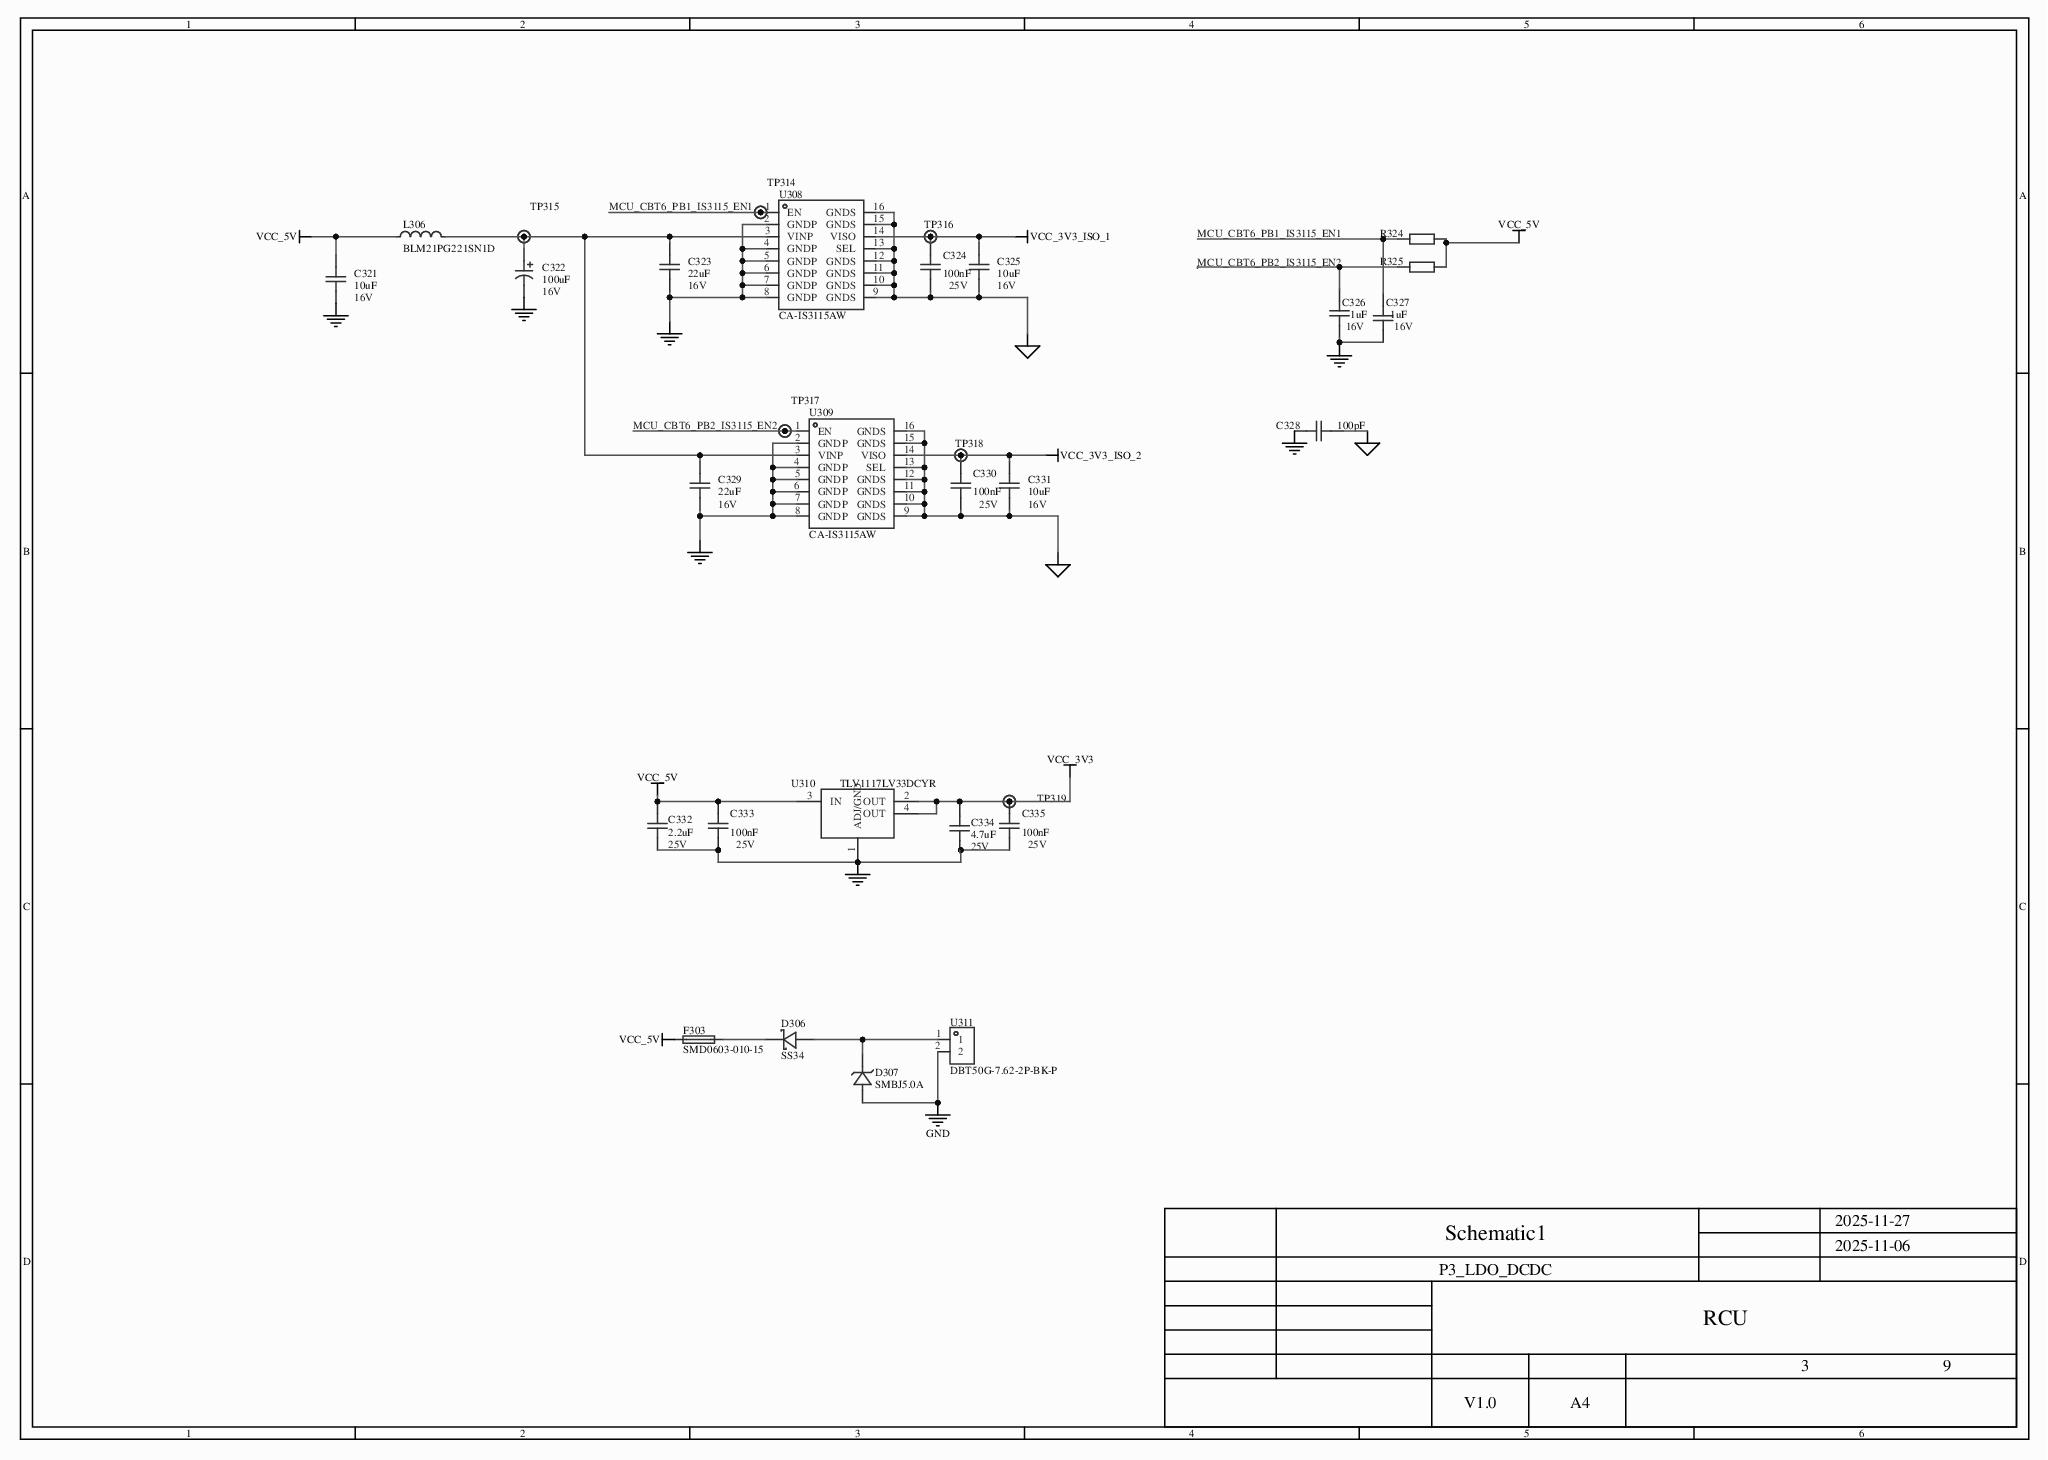
[diagram p0: MISC84429-4.SchDoc]
# Altium project MISC84429-12.PrjPcb (part 2 of 5)
## Sheet MISC84429-4.SchDoc (continued)
### Library data of the parts (continued)
TP314-TP319 = Test-Point: Add into BOM: yes; Symbol: Test-Point; Device: Test-Point; Convert to PCB: yes; Origin Footprint: Test-Point-0.5mm
U308 U309 = CA-IS3115AW: Add into BOM: yes; Output Power: 1.5W; Vin: 5V; Isolation voltage: 5kV; Symbol: CA-IS3115AW; Device: CA-IS3115AW; Supplier Part: C20598894; Manufacturer Part: CA-IS3115AW; Supplier Footprint: SOIC-16-WB; Datasheet: https://item.szlcsc.com/datasheet/CA-IS3115AW/21939206.html; Supplier: LCSC; Convert to PCB: yes; Origin Footprint: SOIC-16_L10.3-W7.5-P1.27-LS10.3-BL
U310 = TLV1117LV33DCYR: Add into BOM: yes; Maximum Input Voltage: 5.5V; Output Voltage: 3.3V; Output Current: 1A; Power Supply Rejection Ratio (PSRR): 75dB@(120Hz); Dropout Voltage: 1.3V@(800mA); standby current: 100uA; Number of Outputs: 1; Symbol: TLV1117LV33DCYR; Device: TLV1117LV33DCYR; Supplier Part: C15578; Manufacturer Part: TLV1117LV33DCYR; Supplier Footprint: SOT-223; Datasheet: https://www.ti.com/cn/lit/gpn/tlv1117lv; Supplier: LCSC; Convert to PCB: yes; Origin Footprint: SOT-223_L6.7-W3.5-P2.30-BR
U311 = DBT50G-7.62-2P-BK-P: Add into BOM: yes; Pitch: 7.62mm; Number of Positions or Pins: 1x2P; Number of PINs Per Row: 2; Current Rating: 20A; Voltage Rating (Max): 300V; Wire Gauge - AWG: 12~22; Symbol: DBT50G-7.62-2P-BK-P; Device: DBT50G-7.62-2P-BK-P; Supplier Part: C496127; Manufacturer Part: DBT50G-7.62-2P-BK-P; Datasheet: https://item.szlcsc.com/datasheet/DBT50G-7.62-2P-BK-P/507694.html; Supplier: LCSC; Convert to PCB: yes; Number of Pins: 2P; Number of Rows: 1; Wire Gauge - mm2: -; Origin Footprint: CONN-TH_2P-P7.62_L15.2-W16.7-EX4.2

## Sheet MISC84429-3.SchDoc
size 431 x 309 mm; Name: Sheet-Symbol; Symbol: Sheet-Symbol; Device: Sheet-Symbol; @Page No: 2; @Page Count: 9; @Schematic Name: 1_P1; @Project Name: Altium_Altium_RCU_2025-11-28_2026-01-14; @Board Name: 1_P1; @Update Date: 2026-01-15; @Create Time: 06:40:55; @Update Time: 14:40:57; @Page Name: 2_P2_POWER; @Create Date: 2026-01-15
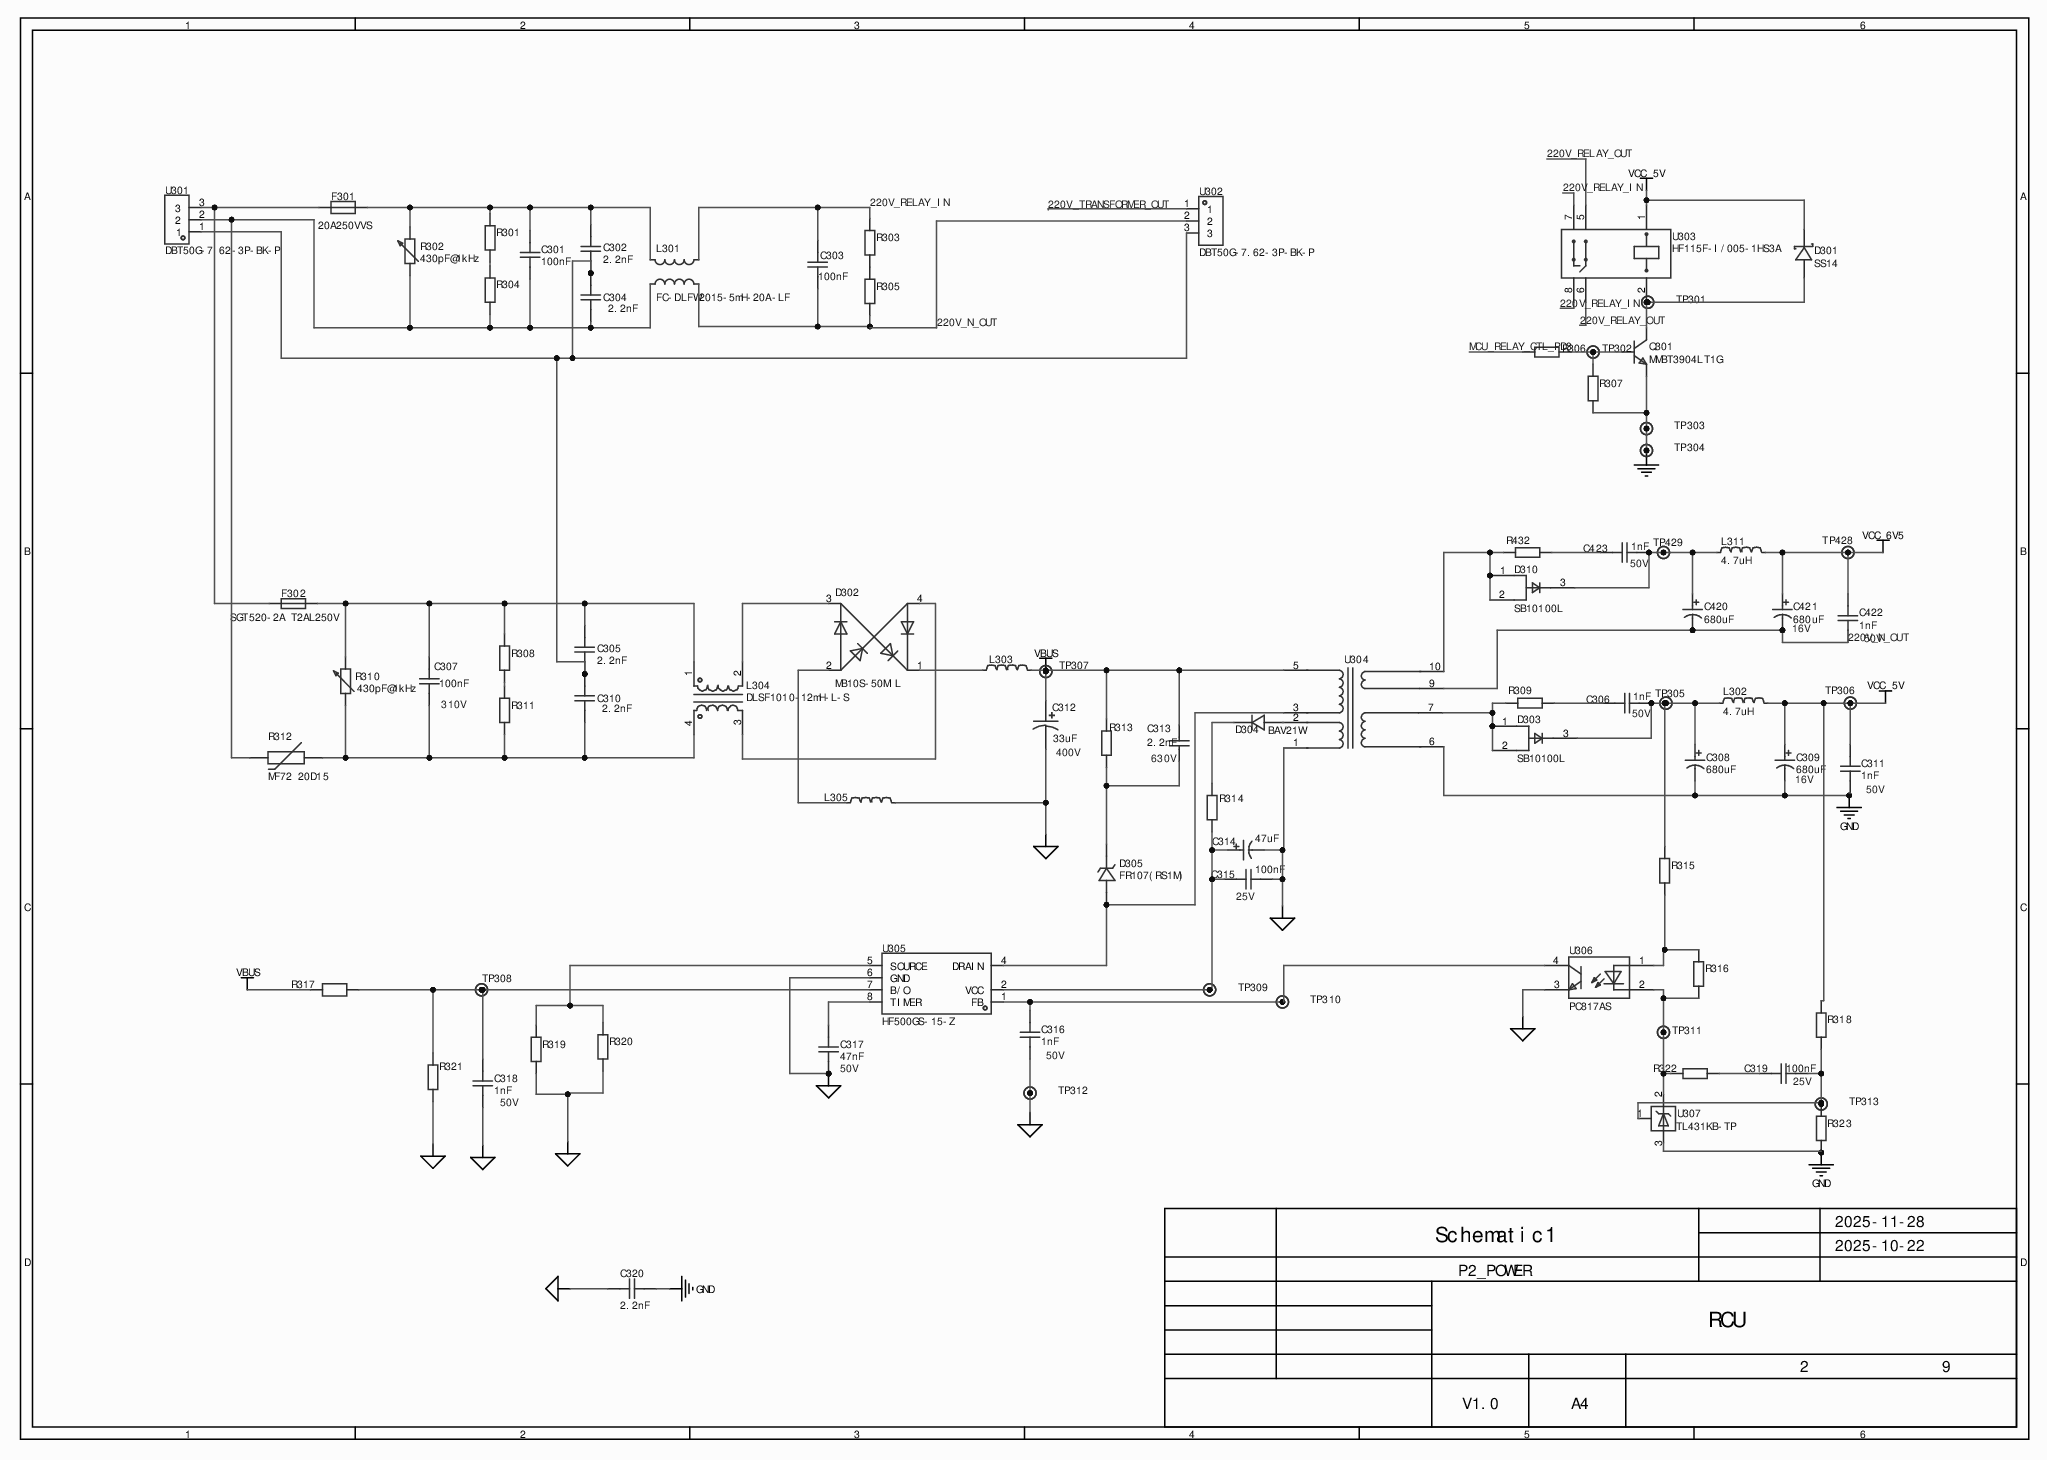
[diagram p1: MISC84429-3.SchDoc]

### Parts
C301  100nF  [CAP-TH_L13.0-W6.0-P10.00-D0.6]
C302  2.2nF  [CAP-TH_L8.0-W4.0-P7.50-D1.2]
C303  100nF  [CAP-TH_L13.0-W6.0-P10.00-D0.6]
C304  2.2nF  [CAP-TH_L8.0-W4.0-P7.50-D1.2]
C305  2.2nF  [CAP-TH_L8.0-W4.0-P7.50-D1.2]
C306  1nF  Voltage Rated: 50V  [C0603]
C307  100nF  Voltage(AC): 310V  [CAP-TH_L13.0-W6.0-P10.00-D0.6]
C308  680uF  [CAP-TH_BD8.0-P3.50-D0.6-FD]
C309  680uF  Voltage Rating: 16V  [CAP-TH_BD8.0-P3.50-D0.6-FD]
C310  2.2nF  [CAP-TH_L8.0-W4.0-P7.50-D1.2]
C311  1nF  Voltage Rated: 50V  [C0603]
C312  33uF  Voltage Rating: 400V  [CAP-TH_BD10.0-P5.00-D1.0-FD]
C313  2.2nF  Voltage Rating: 630V  [C1206]
C314  47uF  [CAP-TH_BD5.0-P2.00-D0.8-FD]
C315  100nF  Voltage Rated: 25V  [C0603]
C316  1nF  Voltage Rated: 50V  [C0603]
C317  47nF  Voltage Rated: 50V  [C0603]
C318  1nF  Voltage Rated: 50V  [C0603]
C319  100nF  Voltage Rated: 25V  [C0603]
C320  2.2nF  [CAP-TH_L10.0-W4.5-P10.00-D0.6-S4.0]
C420  680uF  [CAP-TH_BD8.0-P3.50-D0.6-FD]
C421  680uF  Voltage Rating: 16V  [CAP-TH_BD8.0-P3.50-D0.6-FD]
C422  1nF  Voltage Rated: 50V  [C0603]
C423  1nF  Voltage Rated: 50V  [C0603]
D301  SS14  [SMA_L4.3-W2.6-LS5.2-RD]
D302  MB10S-50MIL  [MBS_L4.7-W3.8-P2.40-LS7.0-TL]
D303  SB10100L  [TO-277A_L4.7-W6.1-LS6.6-TR]
D304  BAV21W  [SOD-123_L2.8-W1.8-LS3.7-RD]
D305  FR107(RS1M)  [SMA_L4.3-W2.6-LS5.2-RD]
D310  SB10100L  [TO-277A_L4.7-W6.1-LS6.6-TR]
F301  20A250VVS  [FUSE-TH_L8.4-W4.0-P5.08-D0.6]
F302  SGT520-2A T2AL250V  [FUSE-SMD_L20.0-W5.0]
L301  FC-DLFW2015-5mH-20A-LF  [FILTER-TH_FC-DLFW2015-5MH-20A-LF]
L302  4.7uH  [IND-SMD_L5.4-W5.2_FXL0530]
L303  (no value)  [L1206]
L304  DLSF1010-12mH-L-S  [IND-TH_4P-L14.0-W12.0_DLSF1010-12MH-L-S]
L305  (no value)  [L1206]
L311  4.7uH  [IND-SMD_L5.4-W5.2_FXL0530]
Q301  MMBT3904LT1G  [SOT-23-3_L2.9-W1.6-P1.90-LS2.8-BR]
R301  (no value)  [R1206]
R302  430pF@1kHz  [RES-TH_L16.5-W5.6-P7.50-D1.2-S3.00]
R303  (no value)  [R1206]
R304  (no value)  [R1206]
R305  (no value)  [R1206]
R306  (no value)  [R0603]
R307  (no value)  [R0603]
R308  (no value)  [R1206]
R309  (no value)  [R1206]
R310  430pF@1kHz  [RES-TH_L16.5-W5.6-P7.50-D1.2-S3.00]
R311  (no value)  [R1206]
R312  MF72 20D15  [RES-TH_L17.5-W6.0-P7.50-D0.8-S7.50]
R313  (no value)  [R1206]
R314  (no value)  [R1206]
R315  (no value)  [R0603]
R316  (no value)  [R0603]
R317  (no value)  [R1206]
R318  (no value)  [R0603]
R319  (no value)  [R1206]
R320  (no value)  [R1206]
R321  (no value)  [R0603]
R322  (no value)  [R0603]
R323  (no value)  [R0603]
R432  (no value)  [R1206]
TP301  (no value)  [Test-Point-0.5mm]
TP302  (no value)  [Test-Point-0.5mm]
TP303  (no value)  [Test-Point-0.5mm]
TP304  (no value)  [Test-Point-0.5mm]
TP305  (no value)  [Test-Point-0.5mm]
TP306  (no value)  [Test-Point-0.5mm]
TP307  (no value)  [Test-Point-0.5mm]
TP308  (no value)  [Test-Point-0.5mm]
TP309  (no value)  [Test-Point-0.5mm]
TP310  (no value)  [Test-Point-0.5mm]
TP311  (no value)  [Test-Point-0.5mm]
TP312  (no value)  [Test-Point-0.5mm]
TP313  (no value)  [Test-Point-0.5mm]
TP428  (no value)  [Test-Point-0.5mm]
TP429  (no value)  [Test-Point-0.5mm]
U301  DBT50G-7.62-3P-BK-P  [CONN-TH_3P-P7.62_L15.2-W24.4-EX4.2]
U302  DBT50G-7.62-3P-BK-P  [CONN-TH_3P-P7.62_L15.2-W24.4-EX4.2]
U303  HF115F-I/005-1HS3A  [RELAY-TH_HF115F-XXX-1HS3]
U304  (no value)  [111]
U305  HF500GS-15-Z  [SOIC-8_7P-L4.9-W3.9-P1.27-LS6.0-BL-PE3]
U306  PC817AS  [SOP-4_L6.5-W4.6-P2.54-LS10.2-TL]
U307  TL431KB-TP  [SOT-23-3_L2.9-W1.4-P1.91-LS2.6-BR]

### Nets
AGND: C312.2 C314.2 C315.2 C316.1 C317.1 C318.1 C320.1 L305.2 R319.1 R320.1 R321.1 TP312.1 U304.1 U305.6(GND) U306.3(CAT)
GND: C308.2 C309.2 C311.1 C320.2 Q301.2 R307.2 R323.1 TP303.1 TP304.1 U304.6 U307.3(-)
VBUS: C312.1 C313.2 L303.2 R313.2 R317.1 TP307.1 U304.5
VCC_5V: C309.1 C311.2 D301.1(K) L302.2 R318.2 TP306.1 U303.1
VCC_6V5: C421.1 C422.2 L311.2 TP428.1
220V_N_OUT: C303.1 C420.2 C421.2 C422.1 L301.4 R305.1 U302.2 U304.9
220V_RELAY_IN: C303.2 L301.3 R303.2 U303.7 U303.8
220V_RELAY_OUT: U303.5 U303.6
220V_TRANSFORMER_OUT: U302.1
MCU_RELAY_CTL_PD3: R306.1
NetC301_1: C301.1 C304.1 L301.1 R302.1 R304.1 R312.1 U301.2
NetC301_2: C301.2 C302.2 F301.2 L301.2 R301.2 R302.2
NetC302_1: C302.1 C304.2 C305.1 C310.2 U301.1 U302.3
NetC305_2: C305.2 C307.2 F302.2 L304.1 R308.2 R310.2
NetC306_1: C306.1 C308.1 D303.3 L302.1 R315.2 TP305.1
NetC306_2: C306.2 R309.2
NetC307_1: C307.1 C310.1 L304.4 R310.1 R311.1 R312.2
NetC313_1: C313.1 D305.1(C) R313.1
NetC314_1: C314.1 C315.1 R314.1 TP309.1 U305.2(VCC)
NetC316_2: C316.2 TP310.1 U305.1(FB) U306.4(AN)
NetC317_2: C317.2 U305.8(TIMER)
NetC318_2: C318.2 R317.2 R321.2 TP308.1 U305.7(B/O)
NetC319_1: C319.1 R322.2
NetC319_2: C319.2 R318.1 R323.2 TP313.1 U307.1(REF)
NetC420_1: C420.1 C423.1 D310.3 L311.1 TP429.1
NetC423_2: C423.2 R432.2
NetD301_2: D301.2(A) Q301.3 TP301.1 U303.2
NetD302_1: D302.1(+) L303.1
NetD302_2: D302.2(-) L305.1
NetD302_3: D302.3(C2) L304.2
NetD302_4: D302.4(C1) L304.3
NetD303_1: D303.1 D303.2 R309.1 U304.7
NetD304_1: D304.1(K) R314.2
NetD304_2: D304.2(A) U304.2
NetD305_2: D305.2(A) U304.3 U305.4(DRAIN)
NetD310_1: D310.1 D310.2 R432.1 U304.10
NetF301_1: F301.1 F302.1 U301.3
NetQ301_1: Q301.1 R306.2 R307.1 TP302.1
NetR301_1: R301.1 R304.2
NetR303_1: R303.1 R305.2
NetR308_1: R308.1 R311.2
NetR315_1: R315.1 R316.2 U306.1(COL)
NetR316_1: R316.1 R322.1 TP311.1 U306.2(EM) U307.2(+)
NetR319_2: R319.2 R320.2 U305.5(SOURCE)

### Notes on the sheet
- 1
- 2
- 3
- 4
- 5
- 6
- A
- B
- C
- D
- Schematic1
- 2025-11-28
- 2025-10-22
- P2_POWER
- RCU
- 9
- V1.0
- A4

### Library data of the parts
C301 C303 C307 = 100nF: Symbol: MPX104K31C3KN15600; Add into BOM: yes; Ratings: X2; Device: 100nF; Supplier Part: C489079; Manufacturer Part: MPX104K31C3KN15600; Datasheet: https://atta.szlcsc.com/upload/public/pdf/source/20200225/C489079_75CB6A5338414DC85C4C6073302579B5.pdf; Supplier: LCSC; Convert to PCB: yes; Value: 100nF; Origin Footprint: CAP-TH_L13.0-W6.0-P10.00-D0.6; Design Item ID: MPX104K31C3KN15600
C302 C304 C305 C310 = 2.2nF: Symbol: G08F1E222MN0B0S0N0; Add into BOM: yes; Voltage(AC): 250V; Ratings: Y2; Device: 2.2nF; Supplier Part: C240878; Manufacturer Part: G08F1E222MN0B0S0N0; Datasheet: https://item.szlcsc.com/datasheet/G08F1E222MN0B0S0N0/239854.html; Supplier: LCSC; Convert to PCB: yes; Value: 2.2nF; Origin Footprint: CAP-TH_L8.0-W4.0-P7.50-D1.2; Design Item ID: G08F1E222MN0B0S0N0
C306 C311 C316 C318 C422 C423 = 1nF: Symbol: GRM188R71H102KA01D; Add into BOM: yes; Temperature Coefficient: X7R; Device: 1nF; Supplier Part: C71653; Manufacturer Part: GRM188R71H102KA01D; Supplier Footprint: 0603; Datasheet: https://atta.szlcsc.com/upload/public/pdf/source/20161108/1478586450384.pdf; Supplier: LCSC; Convert to PCB: yes; Value: 1nF; Origin Footprint: C0603; Design Item ID: GRM188R71H102KA01D
C308 C420 = 680uF: Symbol: ULR687M1CF1ARR; Add into BOM: yes; Voltage Rating: 16V; Ripple Current: 5.1A@100kHz; Pin Spacing: 3.5mm; Device: 680uF; Supplier Part: C248458; Manufacturer Part: ULR687M1CF1ARR; Datasheet: https://atta.szlcsc.com/upload/public/pdf/source/20181106/C248463_8FFE85A6B0231DD342132C712786FADC.pdf; Supplier: LCSC; Convert to PCB: yes; Value: 680uF; Type: -; Diameter: 8mm; Height - Seated (Max): 11.5mm; Origin Footprint: CAP-TH_BD8.0-P3.50-D0.6-FD; Design Item ID: ULR687M1CF1ARR
C309 C421 = 680uF: Symbol: ULR687M1CF1ARR; Add into BOM: yes; Ripple Current: 5.1A@100kHz; Pin Spacing: 3.5mm; Device: 680uF; Supplier Part: C248458; Manufacturer Part: ULR687M1CF1ARR; Datasheet: https://atta.szlcsc.com/upload/public/pdf/source/20181106/C248463_8FFE85A6B0231DD342132C712786FADC.pdf; Supplier: LCSC; Convert to PCB: yes; Value: 680uF; Type: -; Diameter: 8mm; Height - Seated (Max): 11.5mm; Origin Footprint: CAP-TH_BD8.0-P3.50-D0.6-FD; Design Item ID: ULR687M1CF1ARR
C312 = 33uF: Symbol: 87EC0179; Add into BOM: yes; Ripple Current: 440mA@120Hz; Pin Spacing: 5mm; Device: 33uF; Supplier Part: C516822; Manufacturer Part: 87EC0179; Datasheet: https://item.szlcsc.com/datasheet/87EC0179/533670.html; Supplier: LCSC; Convert to PCB: yes; Value: 33uF; Equivalent Series Resistance(ESR): -; Diameter: 10mm; Height - Seated (Max): 18mm; Origin Footprint: CAP-TH_BD10.0-P5.00-D1.0-FD; Design Item ID: 87EC0179
C313 = 2.2nF: Symbol: GRM31BR72J222KW01L; Add into BOM: yes; Temperature Coefficient: X7R; Device: 2.2nF; Supplier Part: C97938; Manufacturer Part: GRM31BR72J222KW01L; Supplier Footprint: 1206; Datasheet: https://item.szlcsc.com/datasheet/GRM31BR72J222KW01L/99147.html; Supplier: LCSC; Convert to PCB: yes; Value: 2.2nF; Origin Footprint: C1206; Design Item ID: GRM31BR72J222KW01L
C314 = 47uF: Symbol: KS476M025D07RR0VH2FP0; Add into BOM: yes; Voltage Rating: 25V; Pin Spacing: 2mm; Device: 47uF; Supplier Part: C44586; Manufacturer Part: KS476M025D07RR0VH2FP0; Datasheet: https://item.szlcsc.com/datasheet/KS476M025D07RR0VH2FP0/45588.html; Supplier: LCSC; Convert to PCB: yes; Value: 47uF; Diameter: 5mm; Height - Seated (Max): 7mm; Origin Footprint: CAP-TH_BD5.0-P2.00-D0.8-FD; Design Item ID: KS476M025D07RR0VH2FP0
C315 C319 = 100nF: Symbol: GRM188R71E104KA01D; Add into BOM: yes; Temperature Coefficient: X7R; Device: 100nF; Supplier Part: C77050; Manufacturer Part: GRM188R71E104KA01D; Supplier Footprint: 0603; Datasheet: https://atta.szlcsc.com/upload/public/pdf/source/20170622/1498103881034.pdf; Supplier: LCSC; Convert to PCB: yes; Value: 100nF; Origin Footprint: C0603; Design Item ID: GRM188R71E104KA01D
C317 = 47nF: Symbol: GCJ188R71H473KA12D; Add into BOM: yes; Temperature Coefficient: X7R; Device: 47nF; Supplier Part: C354386; Manufacturer Part: GCJ188R71H473KA12D; Supplier Footprint: 0603; Datasheet: https://atta.szlcsc.com/upload/public/pdf/source/20190214/C354386_A23112F67A0EA363A33264332A959C51.pdf; Supplier: LCSC; Convert to PCB: yes; Value: 47nF; Origin Footprint: C0603; Design Item ID: GCJ188R71H473KA12D
C320 = 2.2nF: Symbol: AJTF222M2GF0200A082E; Add into BOM: yes; Voltage(AC): 400V; Ratings: Y1; Device: 2.2nF; Supplier Part: C2836435; Manufacturer Part: AJTF222M2GF0200A082E; Datasheet: https://item.szlcsc.com/datasheet/AJTF222M2GF0200A082E/3002607.html; Supplier: LCSC; Convert to PCB: yes; Value: 2.2nF; Origin Footprint: CAP-TH_L10.0-W4.5-P10.00-D0.6-S4.0; Design Item ID: AJTF222M2GF0200A082E
D301 = SS14: Symbol: SS14_C83852; Add into BOM: yes; Voltage - Forward(Vf@If): 500mV@1A; Voltage - DC Reverse(Vr): 40V; Current - Rectified: 1A; Reverse Leakage Current (Ir): 200uA@40V; Non-Repetitive Peak Forward Surge Current: 40A; Device: SS14; Supplier Part: C83852; Manufacturer Part: SS14; Supplier Footprint: SMA(DO-214AC); Datasheet: https://item.szlcsc.com/datasheet/SS14/85019.html; Supplier: LCSC; Convert to PCB: yes; Origin Footprint: SMA_L4.3-W2.6-LS5.2-RD; Design Item ID: SS14_C83852
D302 = MB10S-50MIL: Add into BOM: yes; Voltage - Forward(Vf@If): 1.1V@400mA; Voltage - DC Reverse(Vr): 1kV; Current - Rectified: 1A; Reverse Leakage Current (Ir): 5uA@1kV; Non-Repetitive Peak Forward Surge Current: 35A; Symbol: MB10S-50MIL; Device: MB10S-50MIL; Supplier Part: C2488; Manufacturer Part: MB10S-50MIL; Supplier Footprint: MBS; Datasheet: https://item.szlcsc.com/datasheet/MB10S-50MIL/2865.html; Supplier: LCSC; Convert to PCB: yes; Origin Footprint: MBS_L4.7-W3.8-P2.40-LS7.0-TL; Design Item ID: MB10S-50MIL
D303 D310 = SB10100L: Symbol: SB10100L_C113946; Add into BOM: yes; Voltage - Forward(Vf@If): 850mV@10A; Voltage - DC Reverse(Vr): 100V; Current - Rectified: 10A; Reverse Leakage Current (Ir): 300uA@100V; Non-Repetitive Peak Forward Surge Current: 150A; Device: SB10100L; Supplier Part: C113946; Manufacturer Part: SB10100L; Supplier Footprint: TO-277; Datasheet: https://item.szlcsc.com/datasheet/SB10100L/115185.html; Supplier: LCSC; Convert to PCB: yes; Origin Footprint: TO-277A_L4.7-W6.1-LS6.6-TR; Design Item ID: SB10100L_C113946
D304 = BAV21W: Symbol: BAV21W_C113947; Add into BOM: yes; Voltage - Forward(Vf@If): 1.25V@200mA; Voltage - DC Reverse(Vr): 250V; Current - Rectified: 200mA; Pd - Power Dissipation: 500mW; Reverse Leakage Current (Ir): 100nA@250V; Reverse Recovery Time (trr): 50ns; Non-Repetitive Peak Forward Surge Current: 3A; Device: BAV21W; LCSC Part Name: BAV21W; Supplier Part: C113947; Manufacturer Part: BAV21W; Supplier Footprint: SOD-123; Datasheet: https://item.szlcsc.com/datasheet/BAV21W/115186.html; Supplier: LCSC; Convert to PCB: yes; Origin Footprint: SOD-123_L2.8-W1.8-LS3.7-RD; Design Item ID: BAV21W_C113947
D305 = FR107(RS1M): Add into BOM: yes; Voltage - Forward(Vf@If): 1.3V@1A; Voltage - DC Reverse(Vr): 1kV; Current - Rectified: 1A; Reverse Leakage Current (Ir): 5uA; Reverse Recovery Time (trr): 500ns; Non-Repetitive Peak Forward Surge Current: 30A; Symbol: FR107(RS1M); Device: FR107(RS1M); Supplier Part: C489136; Manufacturer Part: FR107(RS1M); Supplier Footprint: DO-214AC(SMA); Datasheet: https://item.szlcsc.com/datasheet/FR107(RS1M)/499160.html; Supplier: LCSC; Convert to PCB: yes; Operating Junction Temperature Range: -; Origin Footprint: SMA_L4.3-W2.6-LS5.2-RD; Design Item ID: FR107(RS1M)
F301 = 20A250VVS: Symbol: MTS2200A; Add into BOM: yes; Current Rating: 20A; Voltage Rating (DC): 250V; Melting I2t: 960; Interrupt Rating: 35A@250VAC; Pitch: 5.08mm; Device: 20A250VVS; Supplier Part: C2762416; Manufacturer Part: 20A250VVS; Datasheet: https://item.szlcsc.com/datasheet/MTS2200A/2889372.html; Supplier: LCSC; Convert to PCB: yes; Origin Footprint: FUSE-TH_L8.4-W4.0-P5.08-D0.6; Design Item ID: MTS2200A
F302 = SGT520-2A T2AL250V: Add into BOM: yes; Current Rating: 2A; Voltage Rating (AC): 250V; Interrupt Rating: 35A@250VAC; Symbol: SGT520-2A T2AL250V; Device: SGT520-2A T2AL250V; Supplier Part: C2997153; Manufacturer Part: SGT520-2A T2AL250V; Supplier Footprint: D5xL20mm; Datasheet: https://atta.szlcsc.com/upload/public/pdf/source/20220512/3B2013244E644EF8C6E398858F77344C.pdf; Supplier: LCSC; Convert to PCB: yes; Origin Footprint: FUSE-SMD_L20.0-W5.0; Design Item ID: SGT520-2A T2AL250V
L301 = FC-DLFW2015-5mH-20A-LF: Add into BOM: yes; Number of Lines: 2; Withstanding Voltage: 1.5kV; Current Rating: 20A; Inductance @ Frequency: 5mH@1KHz; Symbol: FC-DLFW2015-5mH-20A-LF; Device: FC-DLFW2015-5mH-20A-LF; Supplier Part: C28314498; Manufacturer Part: FC-DLFW2015-5mH-20A-LF; Datasheet: https://atta.szlcsc.com/upload/public/pdf/source/20240808/62DBB3E748F582D3D16D94FF73003319.pdf; Supplier: LCSC; Convert to PCB: yes; Voltage Rating: -; Origin Footprint: FILTER-TH_FC-DLFW2015-5MH-20A-LF; Design Item ID: FC-DLFW2015-5mH-20A-LF
L302 L311 = 4.7uH: Symbol: FXL0530-4R7-M; Add into BOM: yes; Current Rating: 4.5A; Current - Saturation(Isat): 5A; Device: 4.7uH; Supplier Part: C177246; Manufacturer Part: FXL0530-4R7-M; Supplier Footprint: SMD,5.4x5.2mm; Datasheet: https://item.szlcsc.com/datasheet/FXL0530-4R7-M/188638.html; Supplier: LCSC; Convert to PCB: yes; Value: 4.7uH; Origin Footprint: IND-SMD_L5.4-W5.2_FXL0530; Design Item ID: FXL0530-4R7-M
L303 L305 = FCM3216KF-500T05: Add into BOM: yes; Current Rating: 500mA; Number of Circuits: 1; Symbol: FCM3216KF-500T05; Device: FCM3216KF-500T05; Supplier Part: C155098; Supplier Footprint: 1206; Datasheet: https://item.szlcsc.com/datasheet/FCM3216KF-500T05/166440.html; Supplier: LCSC; Convert to PCB: yes; Origin Footprint: L1206; Design Item ID: FCM3216KF-500T05
L304 = DLSF1010-12mH-L-S: Add into BOM: yes; Number of Lines: 2; Voltage Withstand: 1.5kV@AC,1mins; Inductance @ Frequency: 12mH@1kHz; Symbol: DLSF1010-12mH-L-S; Device: DLSF1010-12mH-L-S; Supplier Part: C2936077; Manufacturer Part: DLSF1010-12mH-L-S; Datasheet: https://item.szlcsc.com/datasheet/DLSF1010-12mH-L-S/3287820.html; Supplier: LCSC; Convert to PCB: yes; Origin Footprint: IND-TH_4P-L14.0-W12.0_DLSF1010-12MH-L-S; Design Item ID: DLSF1010-12mH-L-S
Q301 = MMBT3904LT1G: Add into BOM: yes; type: NPN; Current - Collector(Ic): 200mA; Collector - Emitter Voltage VCEO: 40V; Pd - Power Dissipation: 225mW; DC Current Gain: 40@0.1mA,1.0V; Transition frequency(fT): 300MHz; Current - Collector Cutoff: 50nA; Vce Saturation(VCE(sat)): 200mV; Symbol: MMBT3904LT1G; Device: MMBT3904LT1G; Supplier Part: C81464; Manufacturer Part: MMBT3904LT1G; Supplier Footprint: SOT-23; Datasheet: https://item.szlcsc.com/datasheet/MMBT3904LT1G/82615.html; Supplier: LCSC; Convert to PCB: yes; Origin Footprint: SOT-23-3_L2.9-W1.6-P1.90-LS2.8-BR; Design Item ID: MMBT3904LT1G
R301 R303-R305 R308 R311 = RC1206FR-07470KL: Add into BOM: yes; Power(Watts): 250mW; Voltage-Supply(Max): 200V; Symbol: RC1206FR-07470KL; Device: RC1206FR-07470KL; Supplier Part: C137273; Manufacturer Part: RC1206FR-07470KL; Supplier Footprint: 1206; Datasheet: https://item.szlcsc.com/datasheet/RC1206FR-07470KL/148589.html; Supplier: LCSC; Convert to PCB: yes; Origin Footprint: R1206; Design Item ID: RC1206FR-07470KL
R302 R310 = 430pF@1kHz: Symbol: 471KD14; Add into BOM: yes; Varistor Voltage: 470V; Clamping Voltage: 775V; Maximum DC Volts: 385V; Maximum AC Volts: 300V; Peak Current: 6kA; Energy: 175J; Rated Wattage: 600mW; Device: 430pF@1kHz; Supplier Part: C78353; Manufacturer Part: 471KD14; Datasheet: https://item.szlcsc.com/datasheet/471KD14/79488.html; Supplier: LCSC; Convert to PCB: yes; Value: 430pF@1kHz; Origin Footprint: RES-TH_L16.5-W5.6-P7.50-D1.2-S3.00; Design Item ID: 471KD14
R306 R315 = RC0603FR-071KL: Add into BOM: yes; Power(Watts): 100mW; Voltage-Supply(Max): 75V; Symbol: RC0603FR-071KL; Device: RC0603FR-071KL; Supplier Part: C22548; Manufacturer Part: RC0603FR-071KL; Supplier Footprint: 0603; Datasheet: https://atta.szlcsc.com/upload/public/pdf/source/20180316/70C0E2BDAE7FCC62C531A5A58D202EE1.pdf; Supplier: LCSC; Convert to PCB: yes; Origin Footprint: R0603; Design Item ID: RC0603FR-071KL
R307 = RC0603FR-07100KL: Add into BOM: yes; Power(Watts): 100mW; Overload Voltage (Max): 75V; Symbol: RC0603FR-07100KL; Device: RC0603FR-07100KL; Supplier Part: C14675; Manufacturer Part: RC0603FR-07100KL; Supplier Footprint: 0603; Datasheet: https://atta.szlcsc.com/upload/public/pdf/source/20140324/1457707028752.pdf; Supplier: LCSC; Convert to PCB: yes; Origin Footprint: R0603; Design Item ID: RC0603FR-07100KL
R309 R432 = RC1206FR-0722RL: Add into BOM: yes; Power(Watts): 250mW; Voltage-Supply(Max): 200V; Symbol: RC1206FR-0722RL; Device: RC1206FR-0722RL; Supplier Part: C114943; Manufacturer Part: RC1206FR-0722RL; Supplier Footprint: 1206; Datasheet: https://item.szlcsc.com/datasheet/RC1206FR-0722RL/116187.html; Supplier: LCSC; Convert to PCB: yes; Origin Footprint: R1206; Design Item ID: RC1206FR-0722RL
R312 = MF72 20D15: Add into BOM: yes; Steady State Current (Max): 4A; Thermal Time Constant: 43s; Pitch: 7.5mm; Symbol: MF72 20D15; Device: MF72 20D15; Supplier Part: C110642; Manufacturer Part: MF72 20D15; Datasheet: https://item.szlcsc.com/datasheet/MF72%252020D15/111867.html; Supplier: LCSC; Convert to PCB: yes; _1: -; _2: -; _3: -; _4: -; Power(Watts): -; B Constant Tolerance: -; Origin Footprint: RES-TH_L17.5-W6.0-P7.50-D0.8-S7.50; Design Item ID: MF72 20D15
R313 = RC1206FR-07150KL: Add into BOM: yes; Power(Watts): 250mW; Voltage-Supply(Max): 200V; Symbol: RC1206FR-07150KL; Device: RC1206FR-07150KL; Supplier Part: C114931; Manufacturer Part: RC1206FR-07150KL; Supplier Footprint: 1206; Datasheet: https://item.szlcsc.com/datasheet/RC1206FR-07150KL/116175.html; Supplier: LCSC; Convert to PCB: yes; Origin Footprint: R1206; Design Item ID: RC1206FR-07150KL
R314 = RC1206JR-0710RL: Add into BOM: yes; Power(Watts): 250mW; Voltage-Supply(Max): 200V; Symbol: RC1206JR-0710RL; Device: RC1206JR-0710RL; Supplier Part: C137208; Manufacturer Part: RC1206JR-0710RL; Supplier Footprint: 1206; Datasheet: https://item.szlcsc.com/datasheet/RC1206JR-0710RL/148524.html; Supplier: LCSC; Convert to PCB: yes; Origin Footprint: R1206; Design Item ID: RC1206JR-0710RL
R316 = RK73H1JTTD2001F: Manufacturer: KOA; Add into BOM: yes; Power(Watts): 100mW; Overload Voltage (Max): 75V; Symbol: RK73H1JTTD2001F; Device: RK73H1JTTD2001F; Supplier Part: C160026; Manufacturer Part: RK73H1JTTD2001F; Supplier Footprint: 0603; Datasheet: https://atta.szlcsc.com/upload/public/pdf/source/20190516/C346145_73DC9C40D36D5A63BE57BD2EFB7F1781.pdf; Supplier: LCSC; Convert to PCB: yes; Origin Footprint: R0603; Design Item ID: RK73H1JTTD2001F
R317 = 1206W4F1025T5E: Add into BOM: yes; Power(Watts): 250mW; Overload Voltage (Max): 200V; Symbol: 1206W4F1025T5E; Device: 1206W4F1025T5E; Supplier Part: C422611; Manufacturer Part: 1206W4F1025T5E; Supplier Footprint: 1206; Datasheet: https://atta.szlcsc.com/upload/public/pdf/source/20200306/C422600_1E6D84923E4A46A82E41ADD87F860B5C.pdf; Supplier: LCSC; Convert to PCB: yes; Origin Footprint: R1206; Design Item ID: 1206W4F1025T5E
R318 R322 R323 = RC0603FR-0710KL: as R324 on sheet MISC84429-4; Symbol: RC0603FR-0710KL; Device: RC0603FR-0710KL; Supplier Part: C98220; Manufacturer Part: RC0603FR-0710KL; Supplier Footprint: 0603; Datasheet: https://atta.szlcsc.com/upload/public/pdf/source/20180927/C295883_E8D83085EA81BD7DE0B2B681138C15EE.pdf; Supplier: LCSC; Convert to PCB: yes; Origin Footprint: R0603; Design Item ID: RC0603FR-0710KL
R319 R320 = RC1206FR-073R3L: Add into BOM: yes; Power(Watts): 250mW; Voltage-Supply(Max): 200V; Symbol: RC1206FR-073R3L; Device: RC1206FR-073R3L; Supplier Part: C137283; Manufacturer Part: RC1206FR-073R3L; Supplier Footprint: 1206; Datasheet: https://item.szlcsc.com/datasheet/RC1206FR-073R3L/148599.html; Supplier: LCSC; Convert to PCB: yes; Origin Footprint: R1206; Design Item ID: RC1206FR-073R3L
R321 = RC0603FR-0791KL: Add into BOM: yes; Power(Watts): 100mW; Overload Voltage (Max): 75V; Symbol: RC0603FR-0791KL; Device: RC0603FR-0791KL; Supplier Part: C137671; Manufacturer Part: RC0603FR-0791KL; Supplier Footprint: 0603; Datasheet: https://atta.szlcsc.com/upload/public/pdf/source/20180821/C275644_0D56F95EFF785E7D9A1FEF436B37DA78.pdf; Supplier: LCSC; Convert to PCB: yes; Origin Footprint: R0603; Design Item ID: RC0603FR-0791KL
TP301-TP313 TP428 TP429 = Test-Point: Add into BOM: yes; Symbol: Test-Point; Device: Test-Point; Convert to PCB: yes; Origin Footprint: Test-Point-0.5mm; Design Item ID: Test-Point
U301 U302 = DBT50G-7.62-3P-BK-P: Add into BOM: yes; Pitch: 7.62mm; Number of Positions or Pins: 1x3P; Number of PINs Per Row: 3; Current Rating: 20A; Voltage Rating (Max): 300V; Wire Gauge - AWG: 12~22; Symbol: DBT50G-7.62-3P-BK-P; Device: DBT50G-7.62-3P-BK-P; Supplier Part: C496128; Manufacturer Part: DBT50G-7.62-3P-BK-P; Datasheet: https://item.szlcsc.com/datasheet/DBT50G-7.62-3P-BK-P/507695.html; Supplier: LCSC; Convert to PCB: yes; Number of Pins: 3P; Number of Rows: 1; Wire Gauge - mm2: -; Origin Footprint: CONN-TH_3P-P7.62_L15.2-W24.4-EX4.2; Design Item ID: DBT50G-7.62-3P-BK-P
U303 = HF115F-I/005-1HS3A: Add into BOM: yes; Coil Voltage: 5V; Contact Rating: 16A@250VAC; Coil Rated Power: 400mW; Switching Current(Max): 16A; Operate Time: 15ms; Release Time: 8ms; Symbol: HF115F-I/005-1HS3A; Device: HF115F-I/005-1HS3A; Supplier Part: C2976795; Manufacturer Part: HF115F-I/005-1HS3A; Supplier Footprint: DIP,29x12.7mm; Datasheet: https://item.szlcsc.com/datasheet/HF115F-I%252F005-1HS3A/3385015.html; Supplier: LCSC; Convert to PCB: yes; Number of Pins: 6; Contact Material: AgSnO2; Origin Footprint: RELAY-TH_HF115F-XXX-1HS3; Design Item ID: HF115F-I/005-1HS3A
U304 = EE19: Add into BOM: yes; Symbol: EE19; Device: EE19; Convert to PCB: yes; Origin Footprint: 111; Design Item ID: EE19
U305 = HF500GS-15-Z: Add into BOM: yes; Supply Voltage: 12.5V~24V; Switching Frequency: 25kHz; Breakdown Voltage: 700V; Symbol: HF500GS-15-Z; Device: HF500GS-15-Z; LCSC Part Name: HF500GS-15-Z; Supplier Part: C17657021; Manufacturer Part: HF500GS-15-Z; Supplier Footprint: SOIC-7; Datasheet: https://atta.szlcsc.com/upload/public/pdf/source/20240129/526C548A996ED9C4FF96F6AA824E3F87.pdf; Supplier: LCSC; Convert to PCB: yes; Origin Footprint: SOIC-8_7P-L4.9-W3.9-P1.27-LS6.0-BL-PE3; Design Item ID: HF500GS-15-Z
U306 = PC817AS: Add into BOM: yes; Input type: DC; Voltage - Forward(Vf): 1.2V; Output Current: 50mA; Isolation Voltage(Vrms): 5kV; Reverse Voltage: 6V; Load Voltage: 80V; Number of Outputs: 1; Vce Saturation(VCE(sat)): 200mV@1mA,20mA; Rise time: 4us; Fall time: 3us; Current Transfer Ratio (CTR) Minimum: 80%; Current Transfer Ratio (CTR) Maximum/Saturation Value: 600%; Symbol: PC817AS; Device: PC817AS; Supplier Part: C22375537; Manufacturer Part: PC817AS; Supplier Footprint: SMD-4P; Datasheet: https://item.szlcsc.com/datasheet/PC817AS/23885362.html; Supplier: LCSC; Convert to PCB: yes; Forward Current(If): 50mA; Origin Footprint: SOP-4_L6.5-W4.6-P2.54-LS10.2-TL; Design Item ID: PC817AS
U307 = TL431KB-TP: Add into BOM: yes; Output Voltage: 2.495V~36V; Output Current: 100mA; Symbol: TL431KB-TP; Device: TL431KB-TP; LCSC Part Name: TL431KB-TP; Supplier Part: C3680135; Manufacturer Part: TL431KB-TP; Supplier Footprint: SOT-23; Supplier: LCSC; Convert to PCB: yes; Input Voltage: -; Supply Current: -; Noise - 1/10Hz to 10Hz: -; Noise - 10Hz to 10kHz: -; Origin Footprint: SOT-23-3_L2.9-W1.4-P1.91-LS2.6-BR; Design Item ID: TL431KB-TP

## Sheet MISC84429-2.SchDoc
size 431 x 309 mm; Name: Sheet-Symbol; Symbol: Sheet-Symbol; Device: Sheet-Symbol

### Notes on the sheet
- 1
- 2
- 3
- 4
- 5
- 6
- A
- B
- C
- D
- Schematic1
- 2025-11-24
- 2025-10-11
- P1
- RCU
- 9
- V1.0
- A4